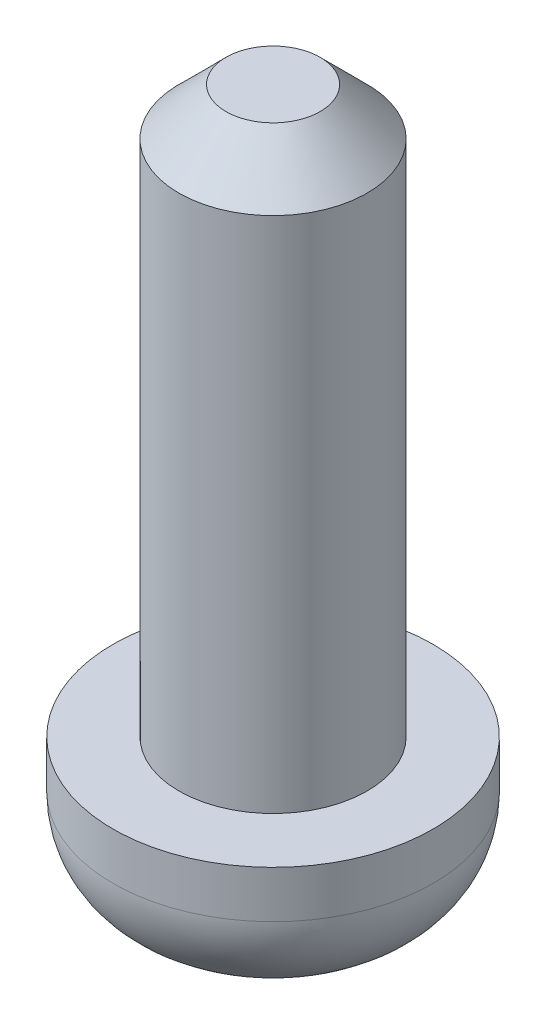
SolidWorks part; units mm, degrees
ref_plane "Front Plane" through (0, 0, 0) normal (0, 0, 1) x (1, 0, 0)
ref_plane "Top Plane" through (0, 0, 0) normal (0, 1, 0) x (1, 0, 0)
ref_plane "Right Plane" through (0, 0, 0) normal (1, 0, 0) x (0, 0, -1)
sketch "Sketch1" plane through (0, 0, 0) normal (0, 1, 0) x (1, 0, 0)
  circle A0 centre (0, 0) radius 1
  dimension "D1" = 2
extrude "Boss-Extrude1" add sketch "Sketch1" along normal blind 6
chamfer "Chamfer1" distance 0.5 angle 45 1 edges at (0, 6, 1)
sketch "Sketch2" plane through (0, 0, 0) normal (0, -1, 0) x (1, 0, 0)
  circle A0 centre (0, 0) radius 1.7
  dimension "D1" = 3.4
extrude "Boss-Extrude2" add sketch "Sketch2" along normal blind 1.5
fillet "Fillet1" radius 1 1 edges at (0, -1.5, -1.7)
